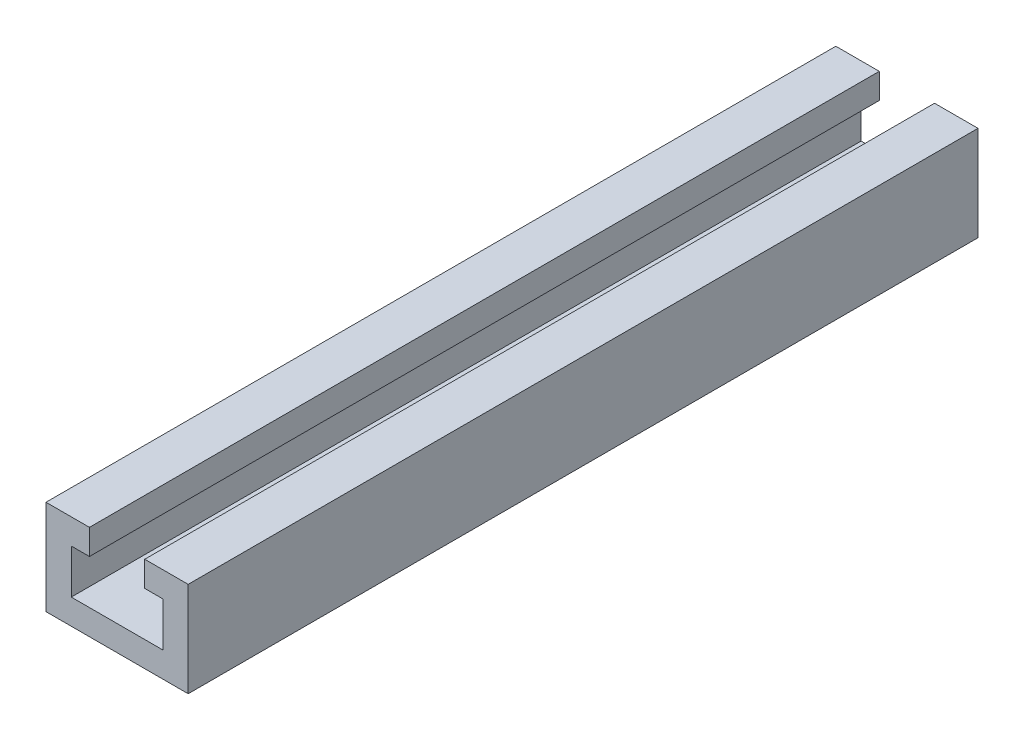
from build123d import *

# Parameters (mm, degrees)
EXTRUDE_1_DEPTH = 25


with BuildPart() as part:
    # 草图1 → 凸台-拉伸1 (new, symmetric)
    with BuildSketch(Plane.XY):
        Polygon((0, 0), (-4.5, 0), (-4.5, 6), (-1.75, 6), (-1.75, 4.4), (-2.9, 4.4), (-2.9, 1.6), (2.9, 1.6), (2.9, 4.4), (1.75, 4.4), (1.75, 6), (4.5, 6), (4.5, 0), align=None)
    extrude(amount=EXTRUDE_1_DEPTH, both=True)


solid = part.part
